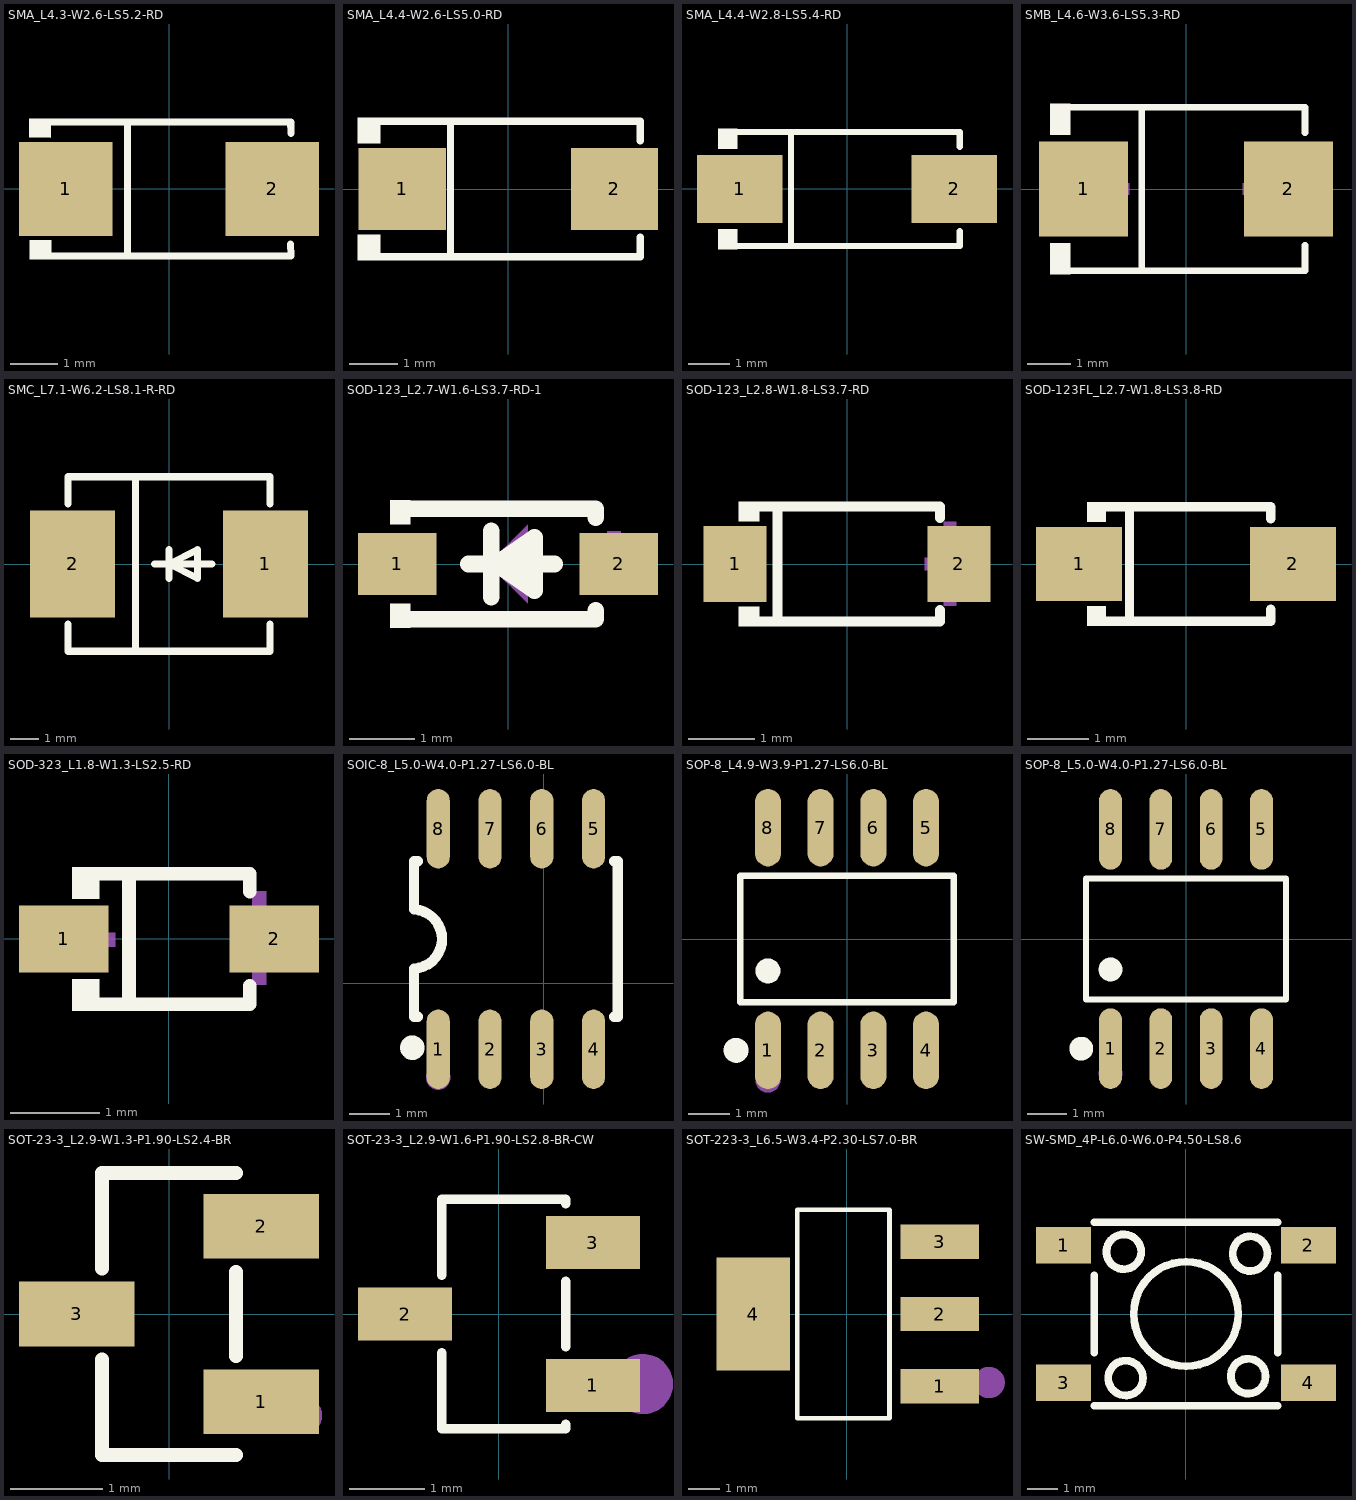
[diagram p0: the footprints below, top view; thin cyan lines are the x and y axes]
# Altium footprint library MISC84402-2.PcbLib: 69 footprints (part 4 of 5)
Each footprint in its own frame and in the unit in brackets; x right, y up, seen from the top. Pads: shape width x height; smd on the part's side, far side on the other; paste and mask are expansions set on the pad; w line width, h text height; cw(c..) or ccw(c..) is an arc to the next point about the centre after c.

## SMA_L4.3-W2.6-LS5.2-RD [mm]
pads (2):
  rect 2x2 smd: 1(-2.2,0) 2(2.2,0)
Top Overlay:
  region: -2.512,-1.096 -2.513,-1.503 -2.973,-1.498 -2.969,-1.096
  region: -2.52,1.502 -2.521,1.096 -2.981,1.1 -2.977,1.502
  lines w0.152: -2.596,-1.426 2.596,-1.426 ; -2.596,1.426 2.596,1.426 2.603,1.187 ; -0.884,-1.426 -0.884,1.426 ; 2.593,-1.176 2.6,-1.415
Mechanical 15:
  region: 2.014,-0.675 2.014,0.675 1.811,0.675 1.811,-0.675
  region: 2.317,-0.101 2.317,0.101 1.507,0.101 1.507,-0.101
  region: -2.317,-0.101 -2.317,0.101 -1.507,0.101 -1.507,-0.101

## SMA_L4.4-W2.6-LS5.0-RD [mm]
pads (2):
  rect 1.8x1.7 smd: 1(-2.192,0) 2(2.192,0)
Top Overlay:
  region: -2.65,1.477 -2.65,0.949 -3.107,0.949 -3.107,1.477
  region: -2.65,-1.477 -2.65,-0.949 -3.107,-0.949 -3.107,-1.477
  lines w0.152: -2.726,-1.401 2.726,-1.401 2.726,-1 ; -2.726,1.401 2.726,1.401 2.726,1 ; -1.197,-1.401 -1.197,1.401
Mechanical 15:
  region: -2.451,-0.099 -2.451,0.099 -1.656,0.099 -1.656,-0.099
  region: 2.451,-0.099 2.451,0.099 1.656,0.099 1.656,-0.099
  region: 2.153,-0.663 2.153,0.663 1.954,0.663 1.954,-0.663

## SMA_L4.4-W2.8-LS5.4-RD [mm]
pads (2):
  rect 2.046x1.62 smd: 1(-2.566,0) 2(2.565,0)
Top Overlay:
  region: -2.625,1.44 -2.625,0.962 -3.082,0.962 -3.082,1.44
  region: -2.625,-1.44 -2.625,-0.962 -3.082,-0.962 -3.082,-1.44
  lines w0.152: -2.701,-1.364 2.701,-1.364 2.701,-1.013 ; -2.701,1.364 2.701,1.364 2.701,1.013 ; -1.339,-1.364 -1.339,1.364
Mechanical 15:
  region: -2.432,-0.097 -2.432,0.097 -1.659,0.097 -1.659,-0.097
  region: 2.432,-0.097 2.432,0.097 1.659,0.097 1.659,-0.097
  region: 2.142,-0.644 2.142,0.644 1.949,0.644 1.949,-0.644

## SMB_L4.6-W3.6-LS5.3-RD [mm]
pads (2):
  rect 2.047x2.192 smd: 1(-2.361,0) 2(2.361,0)
Top Overlay:
  region: -2.668,1.962 -2.668,1.249 -3.125,1.249 -3.125,1.962
  region: -2.668,-1.962 -2.668,-1.249 -3.125,-1.249 -3.125,-1.962
  lines w0.152: -2.744,-1.886 2.744,-1.886 2.744,-1.299 ; -2.744,1.886 2.744,1.886 2.744,1.299 ; -1.016,-1.886 -1.016,1.886
Mechanical 15:
  region: -2.396,-0.136 -2.396,0.136 -1.31,0.136 -1.31,-0.136
  region: 2.396,-0.136 2.396,0.136 1.31,0.136 1.31,-0.136
  region: 1.989,-0.905 1.989,0.905 1.717,0.905 1.717,-0.905

## SMC_L7.1-W6.2-LS8.1-R-RD [mm]
pads (2):
  rect 3.03x3.82 smd: 1(3.435,0) 2(-3.435,0)
Top Overlay:
  lines w0.254: -3.6,-2.141 -3.6,-3.11 3.6,-3.11 3.6,-2.141 ; -3.6,2.141 -3.6,3.11 3.6,3.11 3.6,2.141 ; -1.192,-3.11 -1.192,3.11 ; -0.508,0 1.524,0 ; 0,0.508 0,-0.508 0,0 ; 0,0 1.016,-0.508 1.016,0.508 0,0
Mechanical 15:
  region: 2.54,0.254 4.318,0.254 4.318,-0.254 2.54,-0.254
  region: 3.181,-0.895 3.181,0.883 3.689,0.883 3.689,-0.895
  region: -4.33,0.254 -2.552,0.254 -2.552,-0.254 -4.33,-0.254

## SOD-123_L2.7-W1.6-LS3.7-RD-1 [mm]
pads (2):
  rect 1.2x0.95 smd: 1(-1.7,0) 2(1.7,0)
Top Overlay:
  region: 0.406,-0.406 0.406,0.406 -0.178,0
  region: -1.502,0.977 -1.502,0.607 -1.806,0.607 -1.806,0.977
  region: -1.502,-0.977 -1.502,-0.607 -1.806,-0.607 -1.806,-0.977
  lines w0.254: -1.644,0.849 -1.643,0.85 -1.346,0.85 1.346,0.85 1.346,0.706 ; -1.639,-0.849 -1.638,-0.85 -1.346,-0.85 1.346,-0.85 1.346,-0.706 ; -0.61,0 -0.28,0 ; -0.254,-0.508 -0.254,0.508 ; 0.406,0 0.72,0 ; -0.178,0 0.406,0.406 0.406,-0.406 -0.178,0
Mechanical 15:
  region: 1.19,0.212 2.032,0.212 2.032,0.005 1.189,0.005
  region: 1.525,-0.338 1.525,0.504 1.732,0.504 1.732,-0.339
  region: -2.042,0.124 -1.2,0.124 -1.2,-0.083 -2.042,-0.083
  region: -0.3,0 0.3,-0.6 0.3,0.6

## SOD-123_L2.8-W1.8-LS3.7-RD [mm]
pads (2):
  rect 0.95x1.15 smd: 1(-1.693,0) 2(1.693,0)
Top Overlay:
  region: -1.33,0.942 -1.33,0.647 -1.635,0.647 -1.635,0.942
  region: -1.33,-0.942 -1.33,-0.647 -1.635,-0.647 -1.635,-0.942
  lines w0.152: -1.406,-0.866 1.406,-0.866 1.406,-0.698 ; -1.406,0.866 1.406,0.866 1.406,0.698 ; -1.049,-0.866 -1.049,0.866
Mechanical 15:
  region: -2.03,0.095 -2.03,-0.095 -1.272,-0.095 -1.272,0.095
  region: 1.935,0.098 1.935,-0.092 1.177,-0.092 1.177,0.098
  region: 1.651,0.635 1.651,-0.629 1.461,-0.629 1.461,0.635

## SOD-123FL_L2.7-W1.8-LS3.8-RD [mm]
pads (2):
  rect 1.4x1.2 smd: 1(-1.735,0) 2(1.735,0)
Top Overlay:
  region: -1.3,1.002 -1.3,0.682 -1.605,0.682 -1.605,1.002
  region: -1.3,-1.002 -1.3,-0.682 -1.605,-0.682 -1.605,-1.002
  lines w0.152: -1.376,-0.926 1.376,-0.926 1.376,-0.733 ; -1.376,0.926 1.376,0.926 1.376,0.733 ; -0.917,-0.876 -0.917,0.876
Mechanical 15:
  region: -2.032,0.127 -2.032,-0.065 -1.264,-0.065 -1.264,0.127
  region: 2.035,0.096 2.035,-0.096 1.267,-0.096 1.267,0.096
  region: 1.747,-0.384 1.555,-0.384 1.555,0.384 1.747,0.384

## SOD-323_L1.8-W1.3-LS2.5-RD [mm]
pads (2):
  rect 1x0.75 smd: 1(-1.173,0) 2(1.173,0)
Top Overlay:
  region: -0.775,0.802 -0.775,0.45 -1.08,0.45 -1.08,0.802
  region: -0.775,-0.802 -0.775,-0.45 -1.08,-0.45 -1.08,-0.802
  lines w0.152: -0.851,-0.726 0.901,-0.726 0.901,-0.52 ; -0.851,0.726 0.901,0.726 0.901,0.53 ; -0.447,-0.726 -0.447,0.726
Mechanical 15:
  region: -1.225,0.07 -1.225,-0.086 -0.601,-0.086 -0.601,0.07
  region: 1.315,0.09 1.315,-0.066 0.691,-0.066 0.691,0.09
  region: 1.083,0.53 1.083,-0.51 0.927,-0.51 0.927,0.53

## SOIC-8_L5.0-W4.0-P1.27-LS6.0-BL [mm]
pads (8):
  oval 0.568x1.95 smd: 1(-2.59,-1.623) 2(-1.32,-1.623) 3(-0.05,-1.623) 4(1.22,-1.623) 5(1.22,3.787) 6(-0.05,3.787) 7(-1.32,3.787) 8(-2.59,3.787)
Top Overlay:
  circle w0.3: c-3.225,-1.585 r0.15
  lines w0.254: -3.185,1.809 -3.185,2.582 -3.185,2.987 -3.094,2.987 ; -3.18,1.809 cw(c-3.225,1.082) -3.185,0.356 -3.185,-0.418 -3.185,-0.823 -3.094,-0.823 ; 1.723,-0.823 1.815,-0.823 1.815,-0.418 1.815,2.582 1.815,2.987 1.723,2.987
Mechanical 15:
  circle w0.3: c-2.59,-2.318 r0.15

## SOP-8_L4.9-W3.9-P1.27-LS6.0-BL [mm]
pads (8):
  oval 0.63x1.865 smd: 1(-1.905,-2.682) 2(-0.635,-2.682) 3(0.635,-2.682) 4(1.905,-2.682) 5(1.905,2.683) 6(0.635,2.683) 7(-0.635,2.683) 8(-1.905,2.683)
Top Overlay:
  circle w0.3: c-2.672,-2.682 r0.15
  circle w0.3: c-1.905,-0.769 r0.15
  lines w0.152: -2.576,-1.521 2.576,-1.521 2.576,1.521 -2.576,1.521 -2.576,-1.521
Mechanical 15:
  circle w0.3: c-1.905,-3.4 r0.15

## SOP-8_L5.0-W4.0-P1.27-LS6.0-BL [mm]
pads (8):
  oval 0.574x2.036 smd: 1(-1.905,-2.768) 2(-0.635,-2.768) 3(0.635,-2.768) 4(1.905,-2.768) 5(1.905,2.768) 6(0.635,2.768) 7(-0.635,2.768) 8(-1.905,2.768)
Top Overlay:
  circle w0.3: c-1.905,-0.769 r0.15
  circle w0.3: c-2.644,-2.768 r0.15
  lines w0.152: -2.526,-1.521 -2.526,1.521 2.526,1.521 2.526,-1.521 -2.526,-1.521
Mechanical 15:
  circle w0.3: c-1.905,-3.398 r0.15

## SOT-23-3_L2.9-W1.3-P1.90-LS2.4-BR [mm]
pads (3):
  rect 1.25x0.7 smd: 1(1,-0.95) 2(1,0.95) 3(-1,0)
Top Overlay:
  lines w0.152: -0.726,-0.495 -0.726,-1.526 0.726,-1.526 ; -0.726,0.495 -0.726,1.526 0.726,1.526 ; 0.726,-0.455 0.726,0.455
Mechanical 15:
  circle w0.2: c1.46,-1.1 r0.1

## SOT-23-3_L2.9-W1.6-P1.90-LS2.8-BR-CW [mm]
pads (3):
  rect 1.25x0.7 smd: 1(1.25,-0.95) 2(-1.25,0) 3(1.25,0.95)
Top Overlay:
  lines w0.125: -0.762,-0.517 -0.762,-1.524 0.889,-1.524 0.889,-1.467 ; -0.762,0.517 -0.762,1.524 0.889,1.524 0.889,1.467 ; 0.889,-0.433 0.889,0.433
Mechanical 15:
  circle w0.4: c1.914,-0.931 r0.2

## SOT-223-3_L6.5-W3.4-P2.30-LS7.0-BR [mm]
pads (4):
  rect 2.5x1.1 smd: 1(2.97,-2.3) 2(2.97,0) 3(2.97,2.3)
  rect 2.34x3.6 smd: 4(-2.97,0)
Top Overlay:
  lines w0.152: -1.571,-3.326 -1.571,3.326 1.371,3.326 1.371,-3.326 -1.571,-3.326
Mechanical 15:
  circle w0.5: c4.552,-2.188 r0.25

## SW-SMD_4P-L6.0-W6.0-P4.50-LS8.6 [mm]
pads (4):
  rect 1.8x1.2 smd: 1(-4,2.25) 2(4,2.25) 3(-4,-2.25) 4(4,-2.25)
Top Overlay:
  circle w0.254: c2.032,-2.032 r0.568
  circle w0.254: c2.093,1.971 r0.568
  circle w0.254: c-1.971,-2.093 r0.568
  circle w0.254: c-2.032,2.032 r0.568
  circle w0.254: c0,0 r1.709
  lines w0.254: -3,-3 3,-3 ; -3,-1.269 -3,1.269 ; -3,3 3,3 ; 3,-1.269 3,1.269